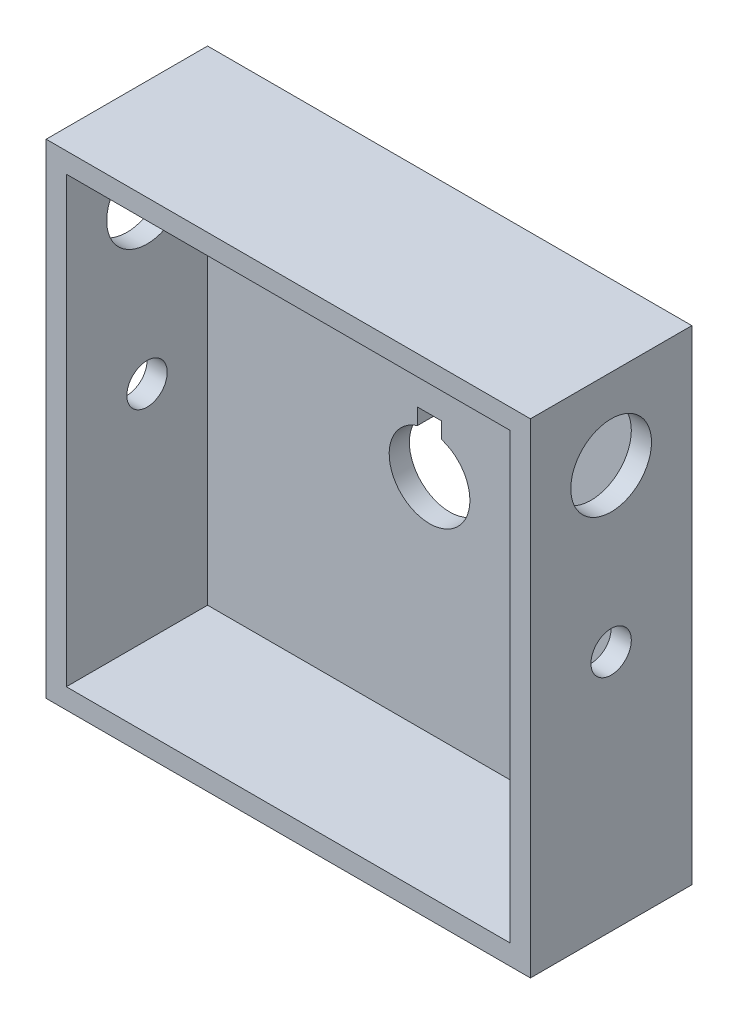
from build123d import *

# Parameters (mm, degrees)
SKETCH_1_W          = 120
SKETCH_1_H          = 120
EXTRUDE_1_DEPTH     = 40
SKETCH_3_R          = 10
SKETCH_3_R_2        = 5
CUT_EXTRUDE_1_DEPTH = 141
SKETCH_4_W          = 110
SKETCH_4_H          = 110
CUT_EXTRUDE_3_DEPTH = 35
CUT_EXTRUDE_4_DEPTH = 94.808315196


with BuildPart() as part:
    # 草图1 → 凸台-拉伸1 (new body)
    with BuildSketch(Plane.XY):
        Rectangle(SKETCH_1_W, SKETCH_1_H)
    extrude(amount=EXTRUDE_1_DEPTH)

    # 草图3 → 切除-拉伸1 (cut, through all)
    with BuildSketch(Plane(origin=(60, 0, 0), x_dir=(0, 0, -1), z_dir=(1, 0, 0))):
        with Locations((-20, 40)):
            Circle(SKETCH_3_R)
        with Locations((-20, 0)):
            Circle(SKETCH_3_R_2)
    extrude(amount=-CUT_EXTRUDE_1_DEPTH, mode=Mode.SUBTRACT)

    # 草图4 → 切除-拉伸3 (cut)
    with BuildSketch(Plane.XY.offset(40)):
        Rectangle(SKETCH_4_W, SKETCH_4_H)
    extrude(amount=-CUT_EXTRUDE_3_DEPTH, mode=Mode.SUBTRACT)

    # 草图5 → 切除-拉伸4 (cut, through all)
    with BuildSketch(Plane(origin=(0, 0, 0), x_dir=(-1, 0, 0), z_dir=(0, 0, -1))):
        with BuildLine():
            Line((-3, 9.539392014), (-3, 13.539392014))
            Line((-3, 13.539392014), (3, 13.539392014))
            Line((3, 13.539392014), (3, 9.539392014))
            ThreePointArc((3, 9.539392014), (0, -10), (-3, 9.539392014))
        make_face()
    extrude(amount=-CUT_EXTRUDE_4_DEPTH, mode=Mode.SUBTRACT)


solid = part.part
